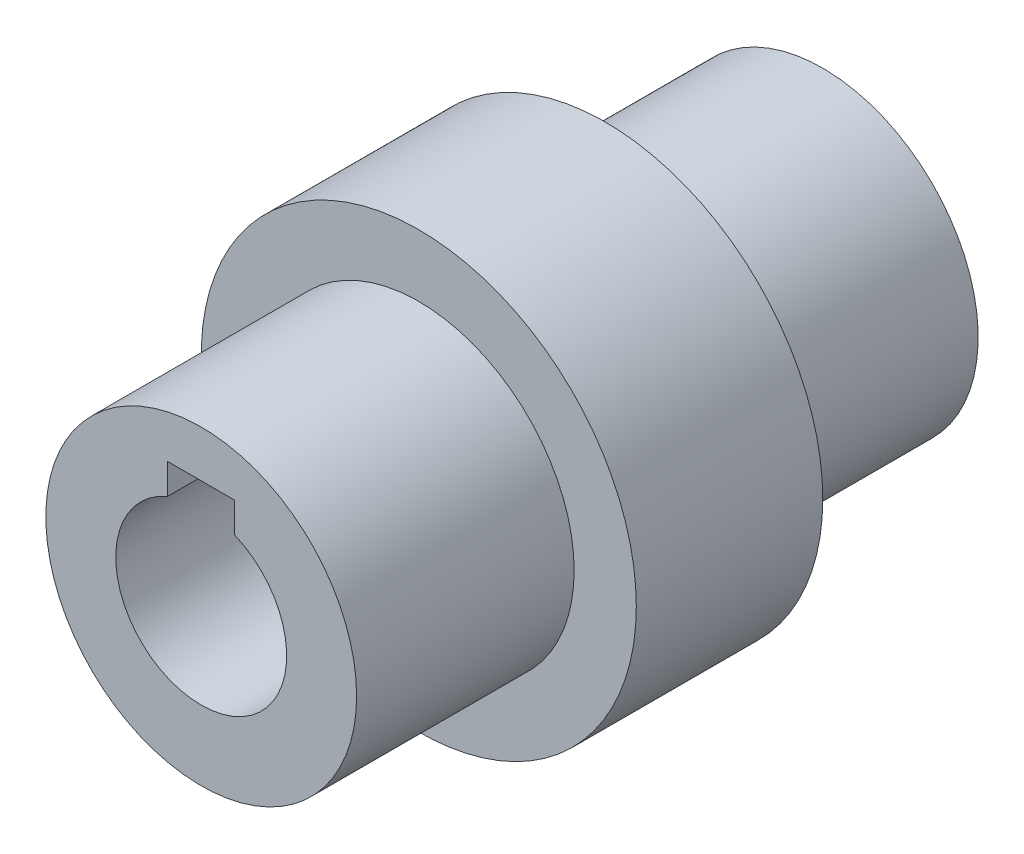
from build123d import *

# Parameters (mm, degrees)
SKETCH_1_R          = 35
EXTRUDE_1_DEPTH     = 15
SKETCH_2_R          = 25
EXTRUDE_2_DEPTH     = 35
EXTRUDE_START       = 35
SKETCH_3_R          = 25
EXTRUDE_3_DEPTH     = 35
CUT_EXTRUDE_1_DEPTH = 25
SKETCH_5_R          = 12.5
CUT_EXTRUDE_2_DEPTH = 25
CUT_EXTRUDE_3_DEPTH = 15


with BuildPart() as part:
    # 草图1 → 凸台-拉伸1 (new, symmetric)
    with BuildSketch(Plane.XY):
        Circle(SKETCH_1_R)
    extrude(amount=EXTRUDE_1_DEPTH, both=True)

    # 草图2 → 凸台-拉伸2 (add)
    with BuildSketch(Plane.XY.offset(15)):
        Circle(SKETCH_2_R)
    extrude(amount=EXTRUDE_2_DEPTH)

    # 草图3 → 凸台-拉伸3 (add)
    with BuildSketch(Plane(origin=(0, 0, -15), x_dir=(-1, 0, 0), z_dir=(0, 0, -1)).offset(EXTRUDE_START)):
        with Locations(Location((0, 0, 0), (0, 0, 180))):
            Circle(SKETCH_3_R)
    extrude(amount=-EXTRUDE_3_DEPTH)

    # 草图4 → 切除-拉伸1 (cut, symmetric)
    with BuildSketch(Plane.XY.offset(50)):
        with BuildLine():
            Line((-5.385, 17.5), (5.385, 17.5))
            Line((5.385, 17.5), (5.385, 12.651651078))
            ThreePointArc((5.385, 12.651651078), (0, -13.75), (-5.385, 12.651651078))
            Line((-5.385, 12.651651078), (-5.385, 17.5))
        make_face()
    extrude(amount=CUT_EXTRUDE_1_DEPTH, both=True, mode=Mode.SUBTRACT)

    # 草图5 → 切除-拉伸2 (cut, symmetric)
    with BuildSketch(Plane(origin=(0, 0, -50), x_dir=(-1, 0, 0), z_dir=(0, 0, -1))):
        Circle(SKETCH_5_R)
    extrude(amount=CUT_EXTRUDE_2_DEPTH, both=True, mode=Mode.SUBTRACT)

    # 草图6 → 切除-拉伸3 (cut, symmetric)
    with BuildSketch(Plane(origin=(0, 0, -50), x_dir=(-1, 0, 0), z_dir=(0, 0, -1))):
        with BuildLine():
            Line((-5, 15), (5, 15))
            Line((5, 15), (5, 11.456439237))
            ThreePointArc((5, 11.456439237), (0, 12.5), (-5, 11.456439237))
            Line((-5, 11.456439237), (-5, 15))
        make_face()
    extrude(amount=CUT_EXTRUDE_3_DEPTH, both=True, mode=Mode.SUBTRACT)


solid = part.part
